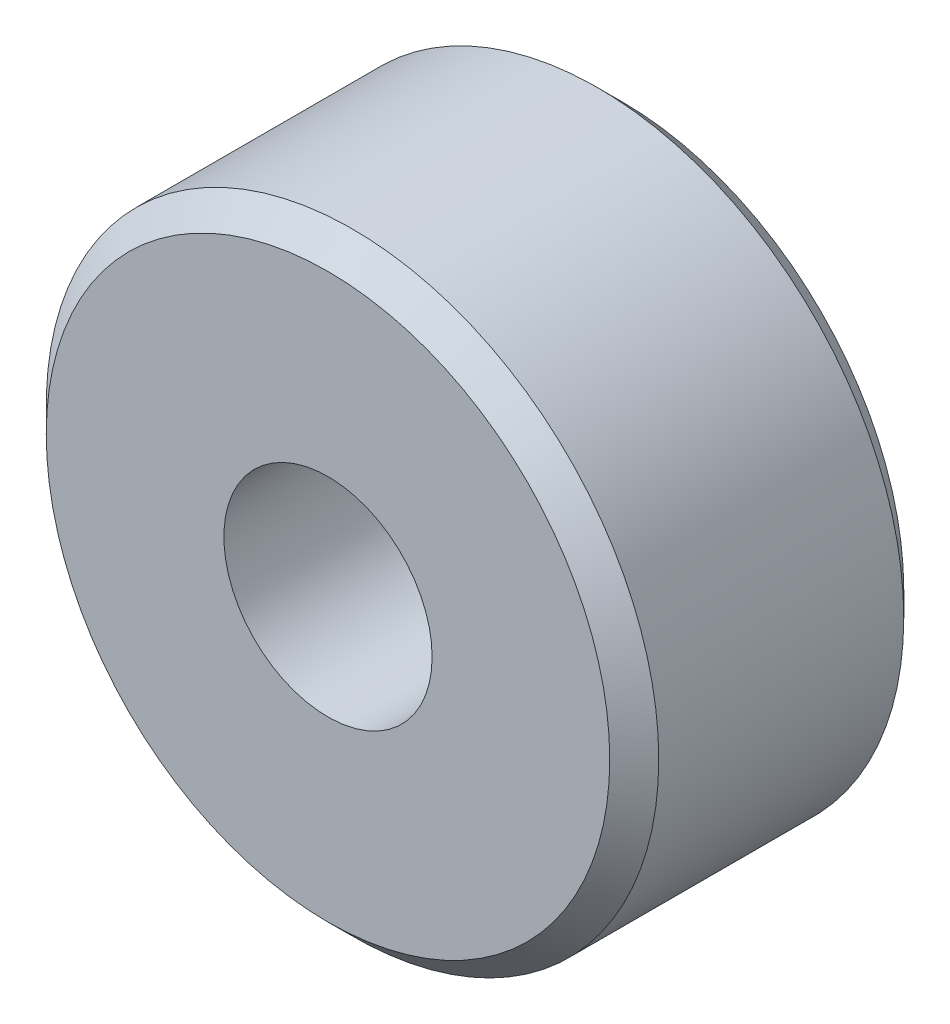
SolidWorks part; units mm, degrees
material "Q235B"
ref_plane "Front Plane" through (0, 0, 0) normal (0, 0, 1) x (1, 0, 0)
ref_plane "Top Plane" through (0, 0, 0) normal (0, 1, 0) x (1, 0, 0)
ref_plane "Right Plane" through (0, 0, 0) normal (1, 0, 0) x (0, 0, -1)
sketch "Sketch1" plane through (0, 0, 0) normal (0, 0, 1) x (1, 0, 0)
  circle A0 centre (0, 0) radius 12.5
  dimension "D1" = 25
extrude "Boss-Extrude1" add sketch "Sketch1" along normal blind 12
hole_wizard "M10 Tapped Hole1" positions "Sketch2" profile "Sketch3" tap size "M10" standard "GB" end condition through all
sketch "Sketch2" plane through (0, 0, 12) normal (0, 0, 1) x (1, 0, 0)
  point P0 (0, 0)
sketch "Sketch3" plane through (0, 0, 12) normal (1, 0, 0) x (0, -1, 0)
  line L0 (0, 0) -> (0, 12)
  line L1 (0, 12) -> (4.25, 12)
  line L2 (4.25, 12) -> (4.25, 0)
  line L5 (4.25, 0) -> (0, 0)
  line L11 (0, -6.35) -> (0, 107.95) construction
  dimension "通孔螺纹孔钻头直径" = 8.5
  dimension "通孔螺纹孔钻头深度" = 12
cosmetic thread "Cosmetic-Thread1" parameters "D2"=10
chamfer "Chamfer1" distance 1 angle 45 2 edges at (12.5, 0, 0) (12.5, 0, 12)
